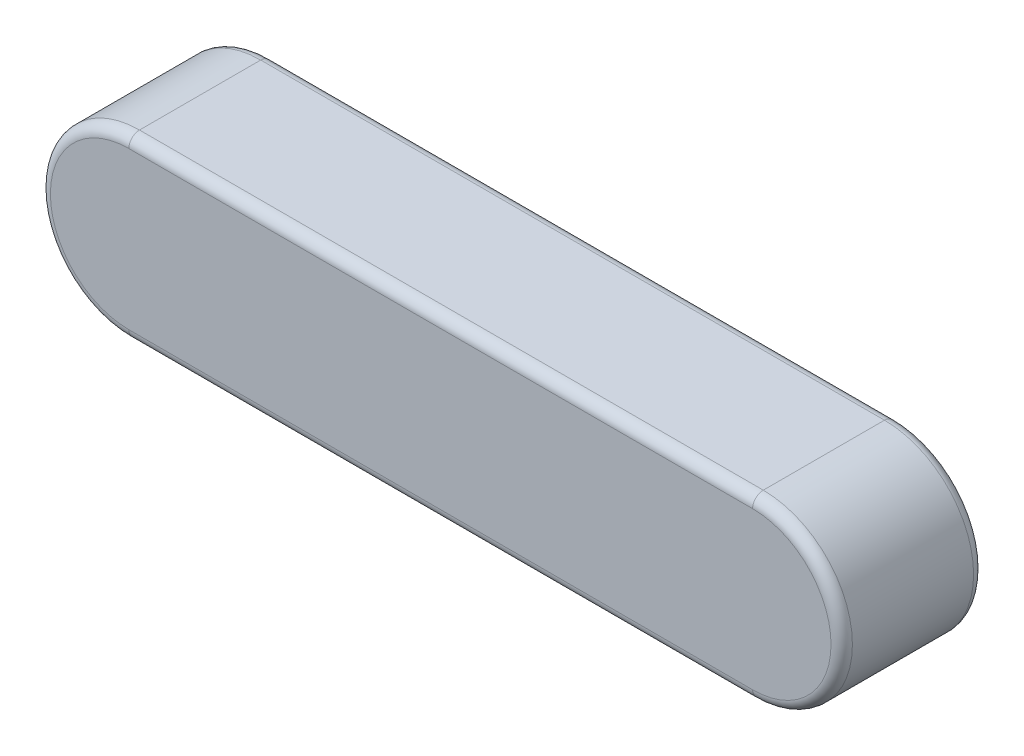
from build123d import *

# Parameters (mm, degrees)
EXTRUDE_512_DEPTH = 8
FILLET_1_R        = 0.6


with BuildPart() as part:
    # 草图1 → Extrude 512 (new body)
    with BuildSketch(Plane.XY):
        with BuildLine():
            Line((-17.5, 5), (17.5, 5))
            ThreePointArc((17.5, 5), (22.5, 0), (17.5, -5))
            Line((17.5, -5), (-17.5, -5))
            ThreePointArc((-17.5, -5), (-22.5, 0), (-17.5, 5))
        make_face()
    extrude(amount=EXTRUDE_512_DEPTH)

    # 圆角1
    fillet_1_edges = [part.edges().sort_by_distance(p)[0] for p in [
        (22.5, 0, 8),
        (0, 5, 8),
        (-22.5, 0, 8),
        (0, 5, 0),
        (22.5, 0, 0),
        (0, -5, 0),
        (-22.5, 0, 0),
        (0, -5, 8),
    ]]
    fillet(fillet_1_edges, radius=FILLET_1_R)


solid = part.part
